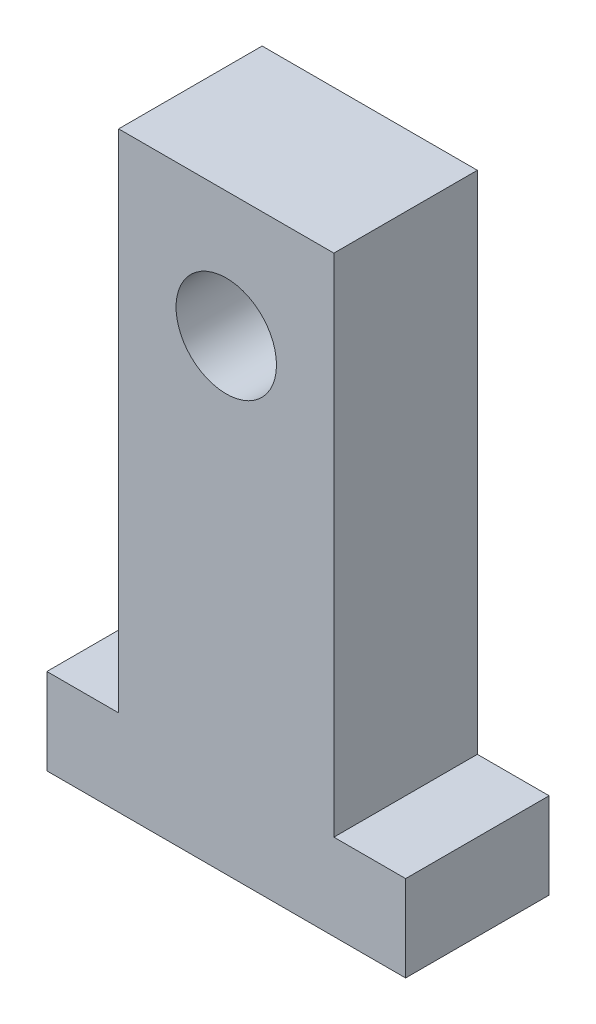
SolidWorks part; units mm, degrees
ref_plane "前视基准面" through (0, 0, 0) normal (0, 0, 1) x (1, 0, 0)
ref_plane "上视基准面" through (0, 0, 0) normal (0, 1, 0) x (1, 0, 0)
ref_plane "右视基准面" through (0, 0, 0) normal (1, 0, 0) x (0, 0, -1)
sketch "草图1" plane through (0, 0, 0) normal (0, 0, 1) x (1, 0, 0)
  line L1 (-25, -41.25) -> (25, -41.25)
  line L2 (-25, -41.25) -> (-25, 41.25)
  line L3 (-25, 41.25) -> (25, 41.25)
  line L4 (25, -41.25) -> (25, 41.25)
  line L5 (-25, -41.25) -> (25, 41.25) construction
  line L6 (-25, 41.25) -> (25, -41.25) construction
  point P0 (0, 0)
  dimension "D1" = 50
  dimension "D2" = 82.5
extrude "凸台-拉伸1" add sketch "草图1" along normal blind 20
sketch "草图2" plane through (0, 0, 20) normal (0, 0, 1) x (1, 0, 0)
  line L0 (0, 0) -> (0, 41.25) construction
  line L1 (25, 41.25) -> (-25, 41.25) construction
  line L2 (-25, -41.25) -> (25, -41.25) construction
  circle A0 centre (0, 23.75) radius 7
  dimension "D1" = 14
  dimension "D2" = 65
extrude "切除-拉伸1" cut sketch "草图2" against normal through all
sketch "草图3" plane through (0, 0, 20) normal (0, 0, 1) x (1, 0, 0)
  line L0 (0, 0) -> (0, 41.25) construction
  line L1 (-25, 41.25) -> (-15, 41.25)
  line L2 (-25, 41.25) -> (-25, -29.25)
  line L3 (-25, -29.25) -> (-15, -29.25)
  line L4 (-15, 41.25) -> (-15, -29.25)
  line L5 (25, 41.25) -> (15, 41.25)
  line L6 (25, 41.25) -> (25, -29.25)
  line L7 (25, -29.25) -> (15, -29.25)
  line L8 (15, 41.25) -> (15, -29.25)
  line L9 (25, 41.25) -> (-25, 41.25) construction
  line L10 (-25, -41.25) -> (25, -41.25) construction
  dimension "D1" = 10
  dimension "D2" = 12
extrude "切除-拉伸2" cut sketch "草图3" against normal through all
